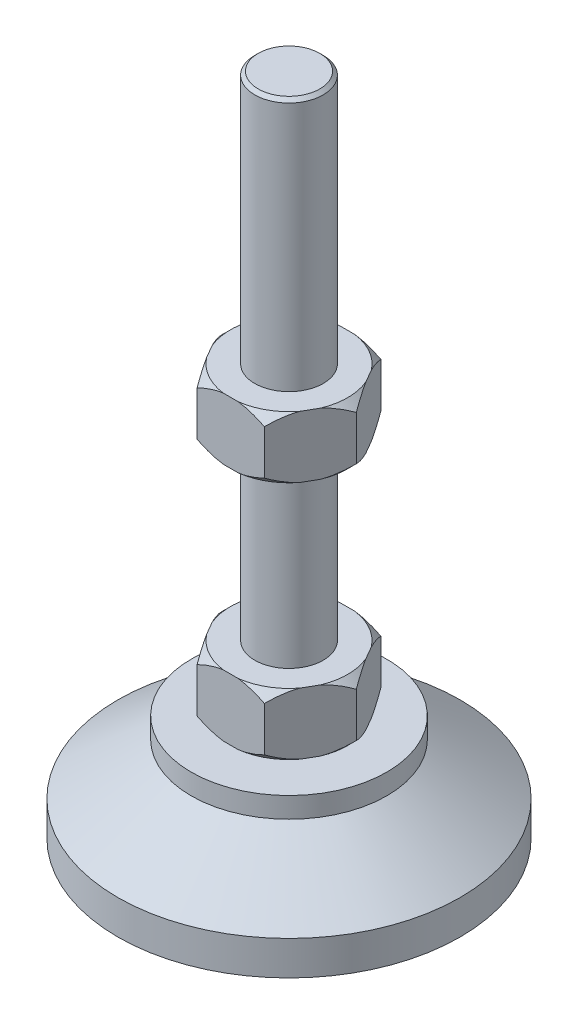
SolidWorks part; units mm, degrees
ref_plane "前视" through (0, 0, 0) normal (0, 0, 1) x (1, 0, 0)
ref_plane "上视" through (0, 0, 0) normal (0, 1, 0) x (1, 0, 0)
ref_plane "右视" through (0, 0, 0) normal (1, 0, 0) x (0, 0, -1)
sketch "草图1" plane through (0, 0, 0) normal (0, 0, 1) x (1, 0, 0)
  line L0 (0, -29.8181) -> (0, 47.3581) construction
  line L1 (10, 169.3407) -> (10, 95.3407)
  line L2 (50, -14.6593) -> (28.5778, 0.3407)
  line L3 (50, -14.6593) -> (50, -24.6593)
  line L4 (50, -24.6593) -> (0, -24.6593)
  line L5 (0, -24.6593) -> (0, 169.3407)
  line L6 (0, 169.3407) -> (10, 169.3407)
  line L7 (28.5778, 0.3407) -> (10, 0.3407)
  line L8 (10, 95.3407) -> (19.65, 95.3407)
  line L9 (10, 7.3407) -> (10, 0.3407)
  line L10 (10, 77.3407) -> (19.65, 77.3407)
  line L11 (19.65, 95.3407) -> (19.65, 77.3407)
  line L12 (10, 25.3407) -> (19.65, 25.3407)
  line L14 (10, 7.3407) -> (19.65, 7.3407)
  line L15 (19.65, 25.3407) -> (19.65, 7.3407)
  line L16 (10, 77.3407) -> (10, 25.3407)
  dimension "D1" = 194
  dimension "D2" = 10
  dimension "D3" = 100
  dimension "D4" = 20
  dimension "D5" = 50
  dimension "D6" = 18
  dimension "D7" = 25
  dimension "D8" = 39.3
  dimension "D9" = 125
  dimension "D10" = 19.65
  dimension "D11" = 18
  dimension "D12" = 120
revolve "旋转1" add sketch "草图1" angle 360 about L0
cosmetic thread "装饰螺纹线1" parameters "D1"=100, "D2"=19
cosmetic thread "装饰螺纹线2" parameters "D1"=100, "D2"=19
sketch "草图2" plane through (0, 0.3407, 0) normal (0, 1, 0) x (1, 0, 0)
  circle A0 centre (0, 0) radius 28.5778
extrude "凸台-拉伸1" add sketch "草图2" along normal blind 6
sketch "草图4" plane through (0, 95.3407, 0) normal (0, 1, 0) x (1, 0, 0)
  line L1 (19.65, 0) -> (9.825, 17.0174)
  line L2 (9.825, 17.0174) -> (-9.825, 17.0174)
  line L3 (-9.825, 17.0174) -> (-19.65, 0)
  line L4 (-19.65, 0) -> (-9.825, -17.0174)
  line L5 (-9.825, -17.0174) -> (9.825, -17.0174)
  line L6 (9.825, -17.0174) -> (19.65, 0)
  circle A0 centre (0, 0) radius 17.0174 construction
  circle A1 centre (0, 0) radius 24.4842
extrude "切除-拉伸5" cut sketch "草图4" against normal blind 88
sketch "草图5" plane through (0, 0, 0) normal (0, 0, 1) x (1, 0, 0)
  line L0 (0, 180.8855) -> (0, -47.3466) construction
  line L1 (-17.15, 95.3407) -> (-19.65, 92.8407)
  line L2 (-19.65, 95.3407) -> (-9.825, 95.3407) construction
  line L3 (-19.65, 77.3407) -> (-19.65, 95.3407) construction
  line L4 (-19.65, 92.8407) -> (-26.9269, 99.1245)
  line L5 (-26.9269, 99.1245) -> (-16.2458, 99.9068)
  line L6 (-16.2458, 99.9068) -> (-17.15, 95.3407)
  line L7 (-17.15, 77.3407) -> (-19.65, 79.8407)
  line L8 (-9.825, 77.3407) -> (-19.65, 77.3407) construction
  line L9 (-19.65, 79.8407) -> (-19.65, 76.2349)
  line L10 (-19.65, 76.2349) -> (-17.15, 77.3407)
  line L11 (-17.15, 25.3407) -> (-19.65, 22.8407)
  line L12 (-19.65, 25.3407) -> (-9.825, 25.3407) construction
  line L13 (-19.65, 7.3407) -> (-19.65, 25.3407) construction
  line L14 (-19.65, 22.8407) -> (-41.601, 16.6236)
  line L15 (-41.601, 16.6236) -> (-25.8403, 26.7626)
  line L16 (-25.8403, 26.7626) -> (-17.15, 25.3407)
  line L17 (-19.65, 9.8407) -> (-17.15, 7.3407)
  line L18 (-19.65, 7.3407) -> (-9.825, 7.3407) construction
  line L19 (-17.15, 7.3407) -> (-28.3675, 7.3407)
  line L20 (-28.3675, 7.3407) -> (-19.65, 9.8407)
  dimension "D1" = 2.5
  dimension "D2" = 2.5
  dimension "D3" = 2.5
  dimension "D4" = 2.5
  dimension "D5" = 2.5
  dimension "D6" = 2.5
  dimension "D7" = 2.5
revolve "切除-旋转1" cut sketch "草图5" angle 360 about L0
chamfer "倒角1" distance 1 angle 45 1 edges at (0, 169.3407, -10)
